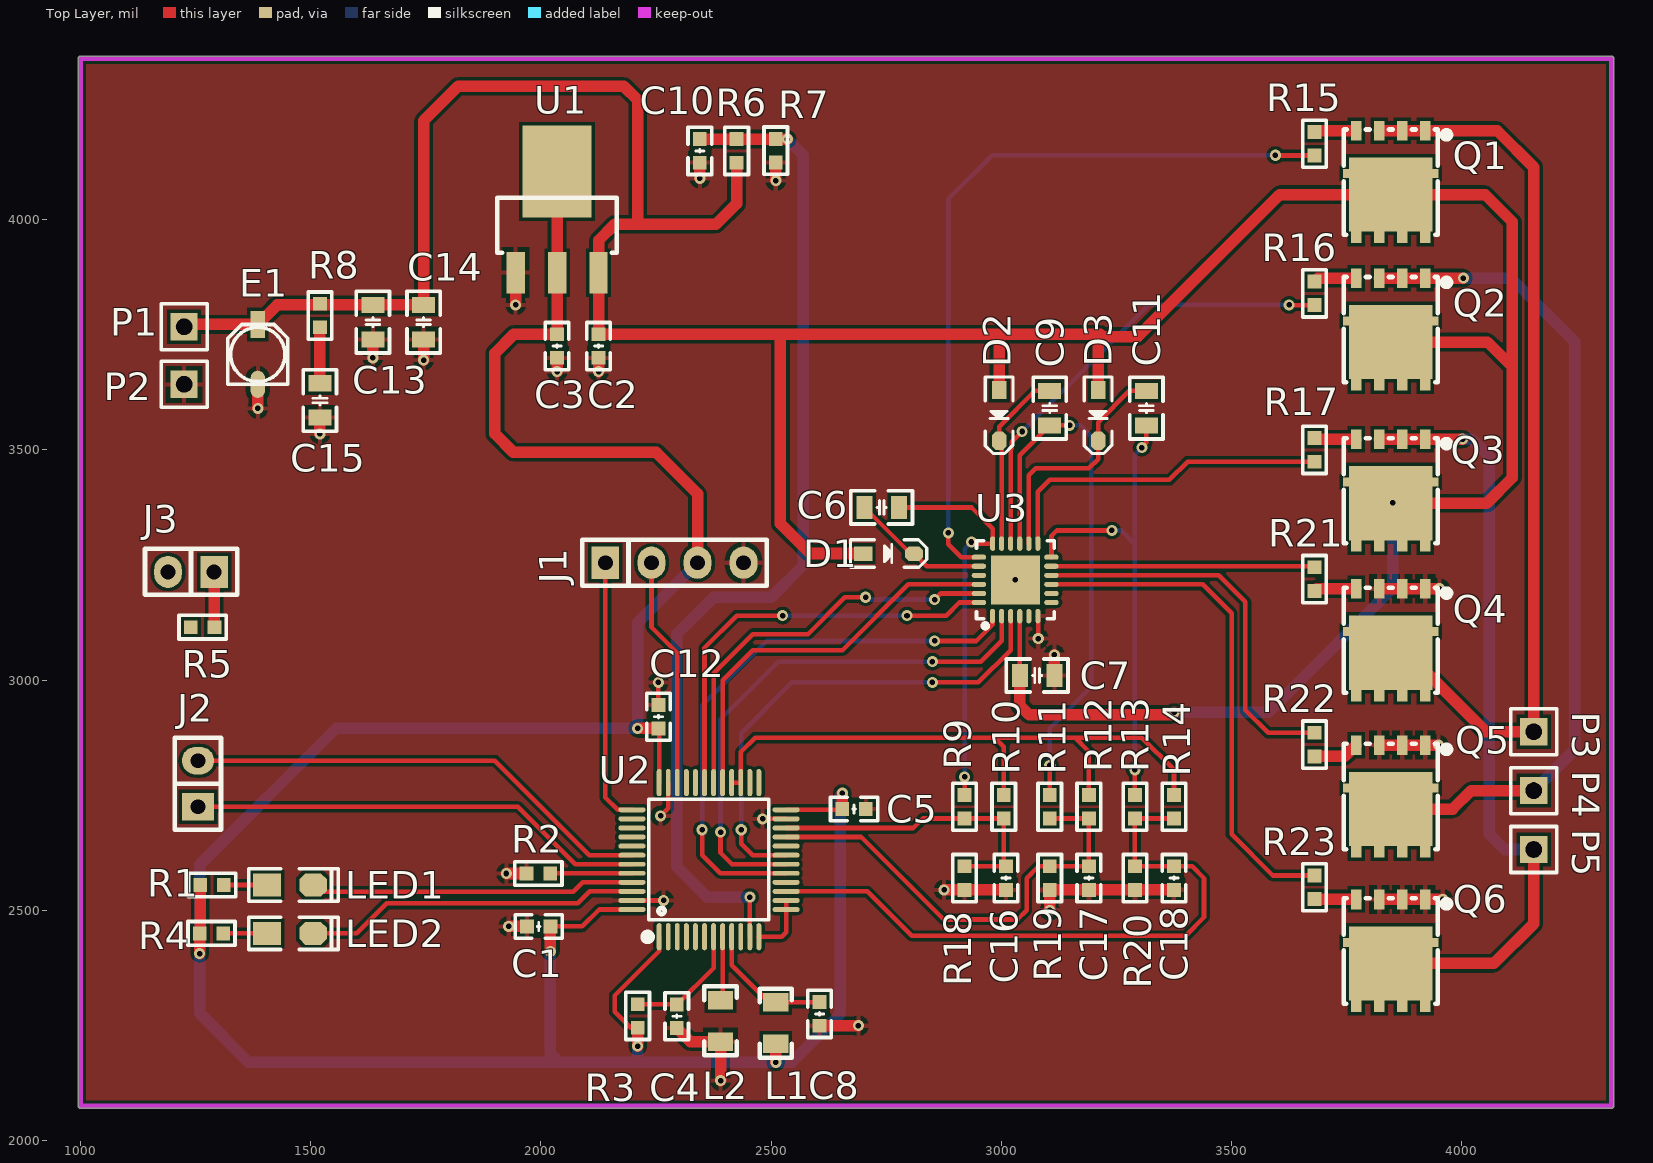
[diagram p0: Top Layer view]
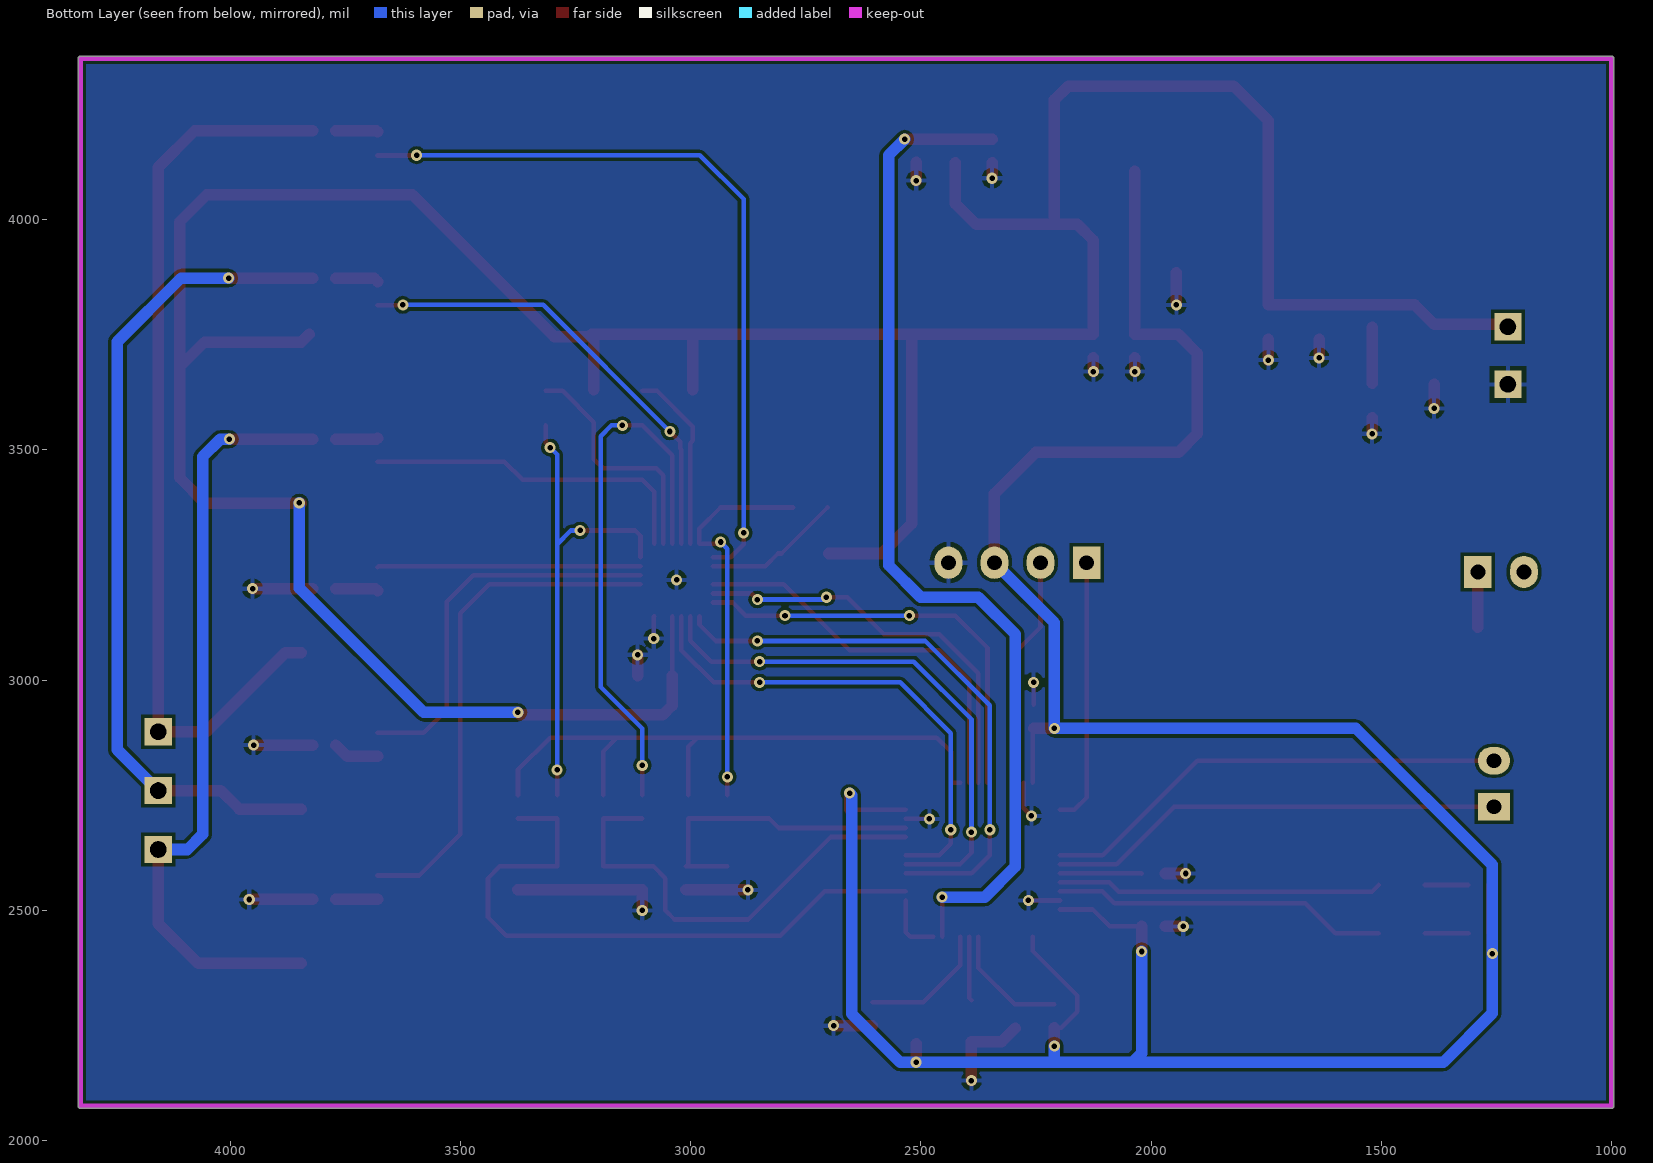
[diagram p1: Bottom Layer view, seen from below]
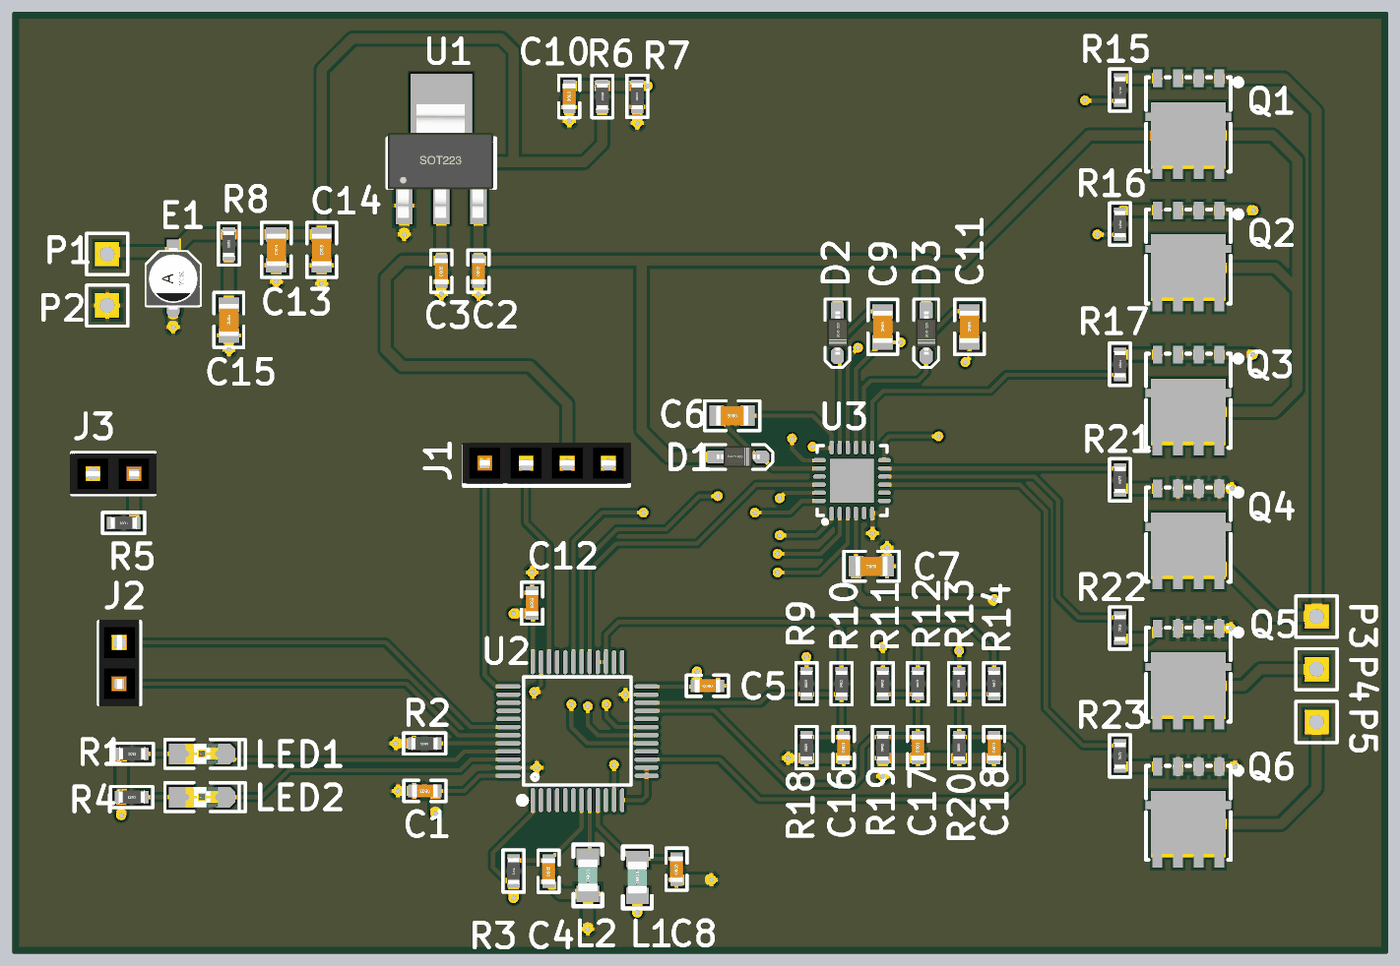
[diagram p2: 3D render of the assembled board from above, using the file's embedded part models]
# Altium PCB MISC82526.PcbDoc
Units mil, origin at the board's own origin, x right, y up, seen from the top; angles counter-clockwise.
Board outline 3335.03 x 2285.03 mil, 2 copper layers (Top Layer, Bottom Layer); 66 components, 53 nets, 254 pads, 58 vias.

## Layer stack, top to bottom (the 12.6 mil dielectric is the usual default, probably not edited)
Top Solder: solder mask 0.4, Solder Resist, Dk 3.5
Top Layer: signal copper 1.4
Dielectric 1: dielectric 12.6, FR-4, Dk 4.8
Bottom Layer: signal copper 1.4
Bottom Solder: solder mask 0.4, Solder Resist, Dk 3.5

## Board outline
1000,2069.99 cw(c1000,2075) 994.99,2075 994.99,4350 cw(c1000,4350) 1000,4355.02 4325,4355.02 cw(c4325,4350) 4330.02,4350 4330.02,2075 cw(c4325,2075) 4325,2069.99

## Design rules (kind name [scope] priority, off if disabled: settings)
Clearance [All] p1: gap=7
MinimumSolderMaskSliver [All] p1: minsoldermaskwidth=0
PolygonConnect [All] p1: connectstyle=Relief reliefconductorwidth=10 reliefentries=4 polygonreliefangle="90 Angle" airgapwidth=10
RoutingVias [All] p1: holewidth=28 width=50 viastyle="Through Hole" minholewidth=28 minwidth=50 maxholewidth=28 maxwidth=50
SilkToSilkClearance [All] p1: silktosilkclearance=0
SilkToSolderMaskClearance [IsPad] p1: minsilkscreentomaskgap=0 clearancetoexposedcopper=TRUE
SolderMaskExpansion [All] p1: expansion=4
Width [All] p1: maxlimit=30 minlimit=10 preferedwidth=10
27 further rules are at their usual default settings.

## Components (designator, comment, footprint, x,y, rotation, side; value= is the part's Value field where it differs from the comment)
C1 "100nF" "C 0603_L" 1995,2465 r180 top
C2 "10uF" "C 0603_L" 2125,3725.59 r90 top
C3 "100nF" "C 0603_L" 2035,3725.59 r90 top
C4 "100nF" "C 0603_L" 2295,2270 r90 top
C5 "100nF" "C 0603_L" 2680,2720 r180 top
C6 "4.7uF" "C 0805_L" 2740,3375 r180 top
C7 "22uF" "C 0805_L" 3077.6,3010 r180 top
C8 "100nF" "C 0603_L" 2605,2275 r90 top
C9 "4.7uF" "C 0805_L" 3105,3590.69 r90 top
C10 "100nF" "C 0603_L" 2345,4149.41 r90 top
C11 "4.7uF" "C 0805_L" 3315,3590.69 r90 top
C12 "100nF" "C 0603_L" 2255,2920.59 r90 top
C13 "22uF" "C 0805_L" 1635,3777.4 r90 top
C14 "22uF" "C 0805_L" 1745,3777.4 r90 top
C15 "10uF" "C 0805_L" 1520,3607.4 r90 top
C16 "100nF" "C 0603_L" 3010,2570 r90 top
C17 "100nF" "C 0603_L" 3190,2570 r90 top
C18 "100nF" "C 0603_L" 3375,2570 r90 top
D1 "B5819WS" SOD-323 2755,3275 r0 top
D2 "B5819WS" SOD-323 2995,3575.12 r270 top
D3 "B5819WS" SOD-323 3210,3575.12 r270 top
E1 "470uF" "CM A(3*5.4)" 1385,3707.4 r90 top
J1 "Female HDR1X4" Fe-HDR1X4/2.54-S 2140,3255 r90 top
J2 "Female HDR1X2" Fe-HDR1X2/2.54-S 1255,2725 r90 top
J3 "XH-2AW" Fe-HDR1X2/2.54-S 1290,3235 r180 top
L1 "10uH" "L 0805" 2510,2255 r90 top
L2 "10uH" "L 0805" 2390,2260 r90 top
LED1 "Red" "LED 0805G" 1455,2555 r0 top
LED2 "Red" "LED 0805G" 1455,2450 r0 top
P1 "HDR1X1" HDR1X1 1225,3767.4 r0 top
P2 "HDR1X1" HDR1X1 1225,3642.4 r0 top
P3 "HDR1X1" HDR1X1 4156.15,2887.87 r270 top
P4 "HDR1X1" HDR1X1 4156.15,2760 r270 top
P5 "HDR1X1" HDR1X1 4156.15,2632.12 r270 top
Q1 "WSD3095DN56" PDFN-8_L5.2-W5.9-P1.27-LS6.2-BL 3855,4085 r180 top
Q2 "WSD3095DN56" PDFN-8_L5.2-W5.9-P1.27-LS6.2-BL 3855,3764.65 r180 top
Q3 "WSD3095DN56" PDFN-8_L5.2-W5.9-P1.27-LS6.2-BL 3855,3414.75 r180 top
Q4 "WSD3095DN56" PDFN-8_L5.2-W5.9-P1.27-LS6.2-BL 3855,3090 r180 top
Q5 "WSD3095DN56" PDFN-8_L5.2-W5.9-P1.27-LS6.2-BL 3855,2750.41 r180 top
Q6 "WSD3095DN56" PDFN-8_L5.2-W5.9-P1.27-LS6.2-BL 3855,2415 r180 top
R1 "1K" "R 0603_L" 1285.59,2555 r180 top
R2 "10K" "R 0603_L" 1994.41,2580 r180 top
R3 "10K" "R 0603_L" 2210,2270.59 r270 top
R4 "2.7K" "R 0603_L" 1284.41,2450 r180 top
R5 "100" "R 0603_L" 1265,3115 r180 top
R6 "47K" "R 0603_L" 2425,4149.41 r270 top
R7 "10K" "R 0603_L" 2510,4150 r90 top
R8 "2" "R 0603_L" 1519.99,3791.82 r90 top
R9 "10K" "R 0603_L" 2920,2725 r90 top
R10 "1K" "R 0603_L" 3005,2725 r90 top
R11 "10K" "R 0603_L" 3105,2725 r90 top
R12 "1K" "R 0603_L" 3190,2725 r90 top
R13 "10K" "R 0603_L" 3290,2725 r90 top
R14 "1K" "R 0603_L" 3375,2725 r90 top
R15 "4.7" "R 0603_L" 3680.01,4165 r270 top
R16 "4.7" "R 0603_L" 3680.01,3840 r270 top
R17 "4.7" "R 0603_L" 3680.01,3500 r270 top
R18 "1K" "R 0603_L" 2920,2570 r90 top
R19 "1K" "R 0603_L" 3105,2570 r90 top
R20 "1K" "R 0603_L" 3290,2570 r90 top
R21 "4.7" "R 0603_L" 3680,3219.41 r90 top
R22 "4.7" "R 0603_L" 3680,2860 r90 top
R23 "4.7" "R 0603_L" 3680,2550 r90 top
U1 "AMS1117" SOT223 2035,3885 r0 top
U2 "CH32V203C8T6" LQFP-48_L7.0-W7.0-P0.50-LS9.0-BL 2365,2610 r0 top
U3 "FD6288Q_C7466367" QFN-24_L4.0-W4.0-P0.50-BL-EP2.7 3030,3210 r0 top

## Footprints (in the part's own frame and the unit in brackets; to place one, negate y for a bottom-side part, rotate by r counter-clockwise, add the part's x,y. Pads: shape width x height; smd on the part's side, far side on the other; paste and mask are expansions set on the pad)
"C 0603_L" [mil] "无极性贴片电容"
  rect 30x30 smd: 1(-25.59,0) 2(25.59,0)
  silkscreen extent -51,-26 51,26, body extent -31,-16 31,16, height 32
"C 0805_L" [mil] "无极性贴片电容"
  rect 35x50 smd: 1(-37.4,0) 2(37.4,0)
  silkscreen extent -67,-36 67,36, body extent -39,-24 39,24, height 20
"CM A(3*5.4)" [mm] "贴片电解电容，直径3mm，高5.4mm"
  rect 1.5x0.8 smd: 1(1.651,0)
  oval 1.5x0.8 smd: 2(-1.65,0)
  silkscreen extent -1.65,-1.65 1.65,1.65, body extent -1.9,-1.65 1.9,1.65, height 5.4
Fe-HDR1X2/2.54-S [mil] "Connector; Header; 2x2 Position"
  rect 60x70 hole 32: 1(0,0)
  oval 60x70 hole 32: 2(100,0)
  silkscreen extent -50,-50 150,50, body extent -55,-48 155,50, height 335
Fe-HDR1X4/2.54-S [mil]
  rect 70x60 hole 32: 1(0,0)
  oval 70x60 hole 32: 2(0,-100) 3(0,-200) 4(0,-300)
  silkscreen extent -50,-350 50,50, body extent -44,-355 54,55, height 335
HDR1X1 [mm]
  rect 1.5x1.5 hole 0.9 slot 0.905 at 0 deg paste+0 mask+0.051: 1(0,0)
  silkscreen extent -1.27,-1.27 1.27,1.27
"L 0805" [mil] "小功率贴片电感"
  rect 40x55 smd: 1(-45,0) 2(45,0)
  silkscreen extent -75,-35 75,35, body extent -39,-24 39,24, height 35
"LED 0805G" [mil] "绿色0805LED"
  rect 60x50 smd: 1(-50,0)
  oct 60x50 smd: 2(50,0)
  silkscreen extent -90,-35 105,35, body extent -39,-25 39,25, height 32
LQFP-48_L7.0-W7.0-P0.50-LS9.0-BL [mm]
  oval 0.27x1.5 smd paste+0 mask+0.051: 1(-2.75,-4.25) 2(-2.25,-4.25) 3(-1.75,-4.25) 4(-1.25,-4.25) 5(-0.75,-4.25) 6(-0.25,-4.25) 7(0.25,-4.25) 8(0.75,-4.25) 9(1.25,-4.25) 10(1.75,-4.25) 11(2.25,-4.25) 12(2.75,-4.25) 25(2.75,4.25) 26(2.25,4.25) 27(1.75,4.25) 28(1.25,4.25) 29(0.75,4.25) 30(0.25,4.25) 31(-0.25,4.25) 32(-0.75,4.25) 33(-1.25,4.25) 34(-1.75,4.25) 35(-2.25,4.25) 36(-2.75,4.25)
  oval 1.5x0.27 smd paste+0 mask+0.051: 13(4.25,-2.75) 14(4.25,-2.25) 15(4.25,-1.75) 16(4.25,-1.25) 17(4.25,-0.75) 18(4.25,-0.25) 19(4.25,0.25) 20(4.25,0.75) 21(4.25,1.25) 22(4.25,1.75) 23(4.25,2.25) 24(4.25,2.75) 37(-4.25,2.75) 38(-4.25,2.25) 39(-4.25,1.75) 40(-4.25,1.25) 41(-4.25,0.75) 42(-4.25,0.25) 43(-4.25,-0.25) 44(-4.25,-0.75) 45(-4.25,-1.25) 46(-4.25,-1.75) 47(-4.25,-2.25) 48(-4.25,-2.75)
  silkscreen extent -3.59,-4.46 3.3,3.34
PDFN-8_L5.2-W5.9-P1.27-LS6.2-BL [mm]
  rect 0.58x1.079 smd paste-100 mask+0.05: 1(-1.668,-2.757) 2(-0.398,-2.757) 3(0.872,-2.757) 4(2.142,-2.757)
  rect 0.58x1.08 smd paste-100 mask+0.05: 5(2.147,2.912) 6(0.878,2.912) 7(-0.392,2.912) 8(-1.662,2.912)
  rect 0.95x0.5 smd paste-100 mask+0.05: 9(-1.932,-0.387) 9(2.407,-0.387)
  rect 4.6x4.1 smd paste-100 mask+0.05: 9(0.237,0.773)
  silkscreen extent -2.96,-2.82 2.84,2.98
QFN-24_L4.0-W4.0-P0.50-BL-EP2.7 [mm]
  oval 0.28x0.8 smd paste+0 mask+0.051: 1(-1.25,-1.803) 2(-0.75,-1.803) 3(-0.25,-1.803) 4(0.25,-1.803) 5(0.75,-1.803) 6(1.25,-1.803) 13(1.25,2.197) 14(0.75,2.197) 15(0.25,2.197) 16(-0.25,2.197) 17(-0.75,2.197) 18(-1.242,2.197)
  oval 0.8x0.28 smd paste+0 mask+0.051: 7(2,-1.053) 8(2,-0.553) 9(2,-0.053) 10(2,0.447) 11(2,0.947) 12(2,1.447) 19(-2,1.447) 20(-2,0.947) 21(-2,0.447) 22(-2,-0.053) 23(-2,-0.553) 24(-2,-1.053)
  rect 2.7x2.7 smd paste+0 mask+0.051: 25(0.012,0.197)
  silkscreen extent -2.14,-2.6 2.16,2.35
"R 0603_L" [mil] "1/10W贴片电阻"
  rect 30x30 smd: 1(-25.59,0) 2(25.59,0)
  silkscreen extent -51,-26 51,26, body extent -31,-16 32,16, height 16
SOD-323 [mm] "1.8x1.3X0.9mm（长宽高，不包括引脚）"
  rect 1x0.8 smd: 1(-1.4,0)
  oct 1x0.8 smd: 2(1.4,0)
  silkscreen extent -2.11,-0.76 2.11,0.76, body extent -1.34,-0.63 1.31,0.67, height 1
SOT223 [mil]
  rect 40x90 smd: 1(-90,0) 2(0,0) 3(90,0)
  rect 150x200 smd: 2(0,220)
  silkscreen extent -130,43 130,163, body extent -130,-30 126,246, height 65

## Part data
C1 C2 C3 C4 C5 C6 C7 C8 C9 C10 C11 C12 C13 C14 C15 C16 C17 C18: library part C, "SMD capacitor"
D1 D2 D3: library part 1N5819, "Schottky diode"
E1: library part CE_SMD, "SMD electrolytic capacitor"
J3: library part "Female HDR1X2"
L1 L2: library part L, "Low-power SMD inductor"
LED1 LED2: library part LED-SMD, "SMD LED"
R1 R2 R3 R4 R5 R6 R7 R8 R9 R10 R11 R12 R13 R14 R15 R16 R17 R18 R19 R20 R21 R22 R23: library part R, "SMD resistor"
U1: "Three-terminal voltage regulator"

## Via types
v1: diameter 24, hole 12, Top Layer to Bottom Layer, 58 vias

## Nets (pads, with @x,y where several pads share a name; then routed paths per layer and width w, separated by ;. In a path a pad name is that pad's centre, name@x,y a point inside that pad or via, vN(x,y) a via of type N, cw(c..) or ccw(c..) an arc to the next point about the centre after c; other vN are vias at no path point)
3.3V: C1.1 C3.2 C5.2 C12.1 J1.3 L1.1 R1.2 R3.2 R4.2 U1.2 U2.1 U2.24 U2.36 U2.48 | length 6444.5
  Top Layer w10: C1.1 2090,2465 2126.73,2501.73 U2.48 ; R3.2 2195,2245 2160,2280 2160,2315 2256.73,2411.73 U2.1 ; C12.1 2256.73,2893.27 U2.36 ; U2.24 2652.68,2718.27 C5.2
  Top Layer w25: v1(1258.82,2406.18) R4.2 1260,2451.18 R1.2 ; v1(2020.59,2410.59) C1.1 ; U1.2@2035,4105 2035,3885 C3.2 1941.18,3751.18 1900,3710 1900,3535 1940,3495 2250,3495 2340,3405 J1.3 ; v1(2210,2205) R3.2 ; v1(2210,2895) C12.1 ; v1(2510,2170) L1.1 ; C5.2 v1(2654.41,2754.41)
  Bottom Layer w25: v1(2020.59,2410.59) 2020.59,2189.41 2040,2170 ; v1(2210,2205) 2210,2175 2205,2170 ; J1.3 2210,3125 v1(2210,2895) 1555,2895 1258.82,2598.82 v1(1258.82,2406.18) 1258.82,2276.18 1365,2170 2040,2170 ; v1(2654.41,2754.41) 2650,2750 2650,2275 2545,2170 v1(2510,2170) 2205,2170 ; 2040,2170 2205,2170
ABMF: C16.2 R9.1 R10.1 R18.2 U2.22 | length 677.1
  Top Layer w10: U2.22 2808.9,2678.9 2829.41,2699.41 R9.1 R10.1 3005,2600.58 C16.2 R18.2
BAT_ADC: C10.2 R6.1 R7.2 U2.11 | length 2243.6
  Top Layer w10: U2.11 v1(2453.58,2528.58)
  Top Layer w25: C10.2 R6.1 v1(2535,4175)
  Bottom Layer w25: v1(2453.58,2528.58) 2361.42,2528.58 2295,2595 2295,3100 2375,3180 2500,3180 2570,3250 2570,4140 v1(2535,4175)
BBMF: C17.2 R11.1 R12.1 R19.2 U2.21 | length 1009.6
  Top Layer w10: U2.21 2695.79,2659.21 2875,2480 3035,2480 3055,2500 3055,2570 3080.59,2595.59 R19.2 C17.2 R12.1 R11.1
CBMF: C18.2 R13.1 R14.1 R20.2 U2.15 | length 1398.5
  Top Layer w10: U2.15 2708.9,2541.1 2805,2445 3400,2445 3440,2485 3440,2570 3414.41,2595.59 C18.2 R20.2 R13.1 R14.1
CLK: J1.1 U2.37 | length 578.8
  Top Layer w10: J1.1 2140,2745 2166.73,2718.27 U2.37
CMPO: U2.12 U2.13 U2.14 | length 132.1
  Top Layer w10: U2.12 2522.68,2442.68 2532.32,2452.32 U2.13 U2.14
DIO: J1.2 U2.34 | length 500.9
  Top Layer w10: J1.2 2240,3115 2296.1,3058.9 U2.34
ERR: LED1.2 U2.45 | length 707.5
  Top Layer w10: LED1.2 1520,2540 2070,2540 2090.79,2560.79 U2.45
GND: C1.2 C2.1 C3.1 C4.1 C5.1 C7.1 C8.1 C10.1 C12.2 C13.1 C14.1 C15.1 C16.1 C17.1 C18.1 E1.2 J1.4 L2.1 P2.1 Q4.1 Q4.2 Q4.3 Q5.1 Q5.2 Q5.3 Q6.1 Q6.2 Q6.3 R2.2 R7.1 R18.1 R19.1 R20.1 U1.1 U2.23 U2.35 U2.47 U3.6 U3.25 | length 1923.2
  Top Layer w10: U2.47 v1(2266.42,2521.42) ; C12.2 v1(2255,2995) ; v1(2260,2705) 2276.42,2721.42 U2.35 ; v1(2481.42,2698.58) U2.23 ; U3.6 3080,3138.24 v1(3080,3090)
  Top Layer w25: v1(1385,3590) E1.2 ; v1(1520,3535) C15.1 ; v1(1635,3700) C13.1 ; v1(1745,3695) C14.1 ; v1(1925,2580) R2.2 ; v1(1930,2465) C1.2 ; v1(1945,3815) U1.1 ; v1(2035,3670) C3.1 ; v1(2125,3670) C2.1 ; C4.1 2324.41,2215 L2.1 v1(2390,2130) ; v1(2345,4090) C10.1 ; v1(2510,4085) R7.1 ; C8.1 v1(2689.41,2249.41) ; v1(2875.59,2544.41) R18.1 C16.1 ; v1(3105,2500) R19.1 C17.1 R20.1 C18.1 ; C7.1 v1(3115,3055) ; Q6.3 Q6.2 Q6.1 v1(3958.55,2523.55) ; Q5.3 Q5.2 Q5.1 v1(3948.96,2858.96) ; Q4.3 Q4.2 Q4.1 v1(3951.45,3198.55)
  other v1: 3030.49,3217.76
HOA: R15.2 U3.19 | length 1662.5
  Top Layer w10: v1(2885,3320) 2885,3295 2913.02,3266.98 U3.19 ; v1(3595,4140) 3595.59,4139.41 R15.2
  Bottom Layer w10: v1(2885,3320) 2885,4045 2980,4140 v1(3595,4140)
HOB: R16.2 U3.16 | length 1002.9
  Top Layer w10: U3.16 3020.17,3500.64 3022.75,3503.22 3022.75,3517.75 v1(3045,3540) ; v1(3625,3815) 3625.59,3814.41 R16.2
  Bottom Layer w10: v1(3045,3540) 3320,3815 v1(3625,3815)
HOC: R17.2 U3.13 | length 740.5
  Top Layer w10: U3.13 3079.22,3409.22 3105,3435 3365,3435 3404.41,3474.41 R17.2
LOA: R21.2 U3.11 | length 572.2
  Top Layer w10: U3.11 3677.71,3247.3 R21.2
LOB: R22.2 U3.10 | length 850.6
  Top Layer w10: U3.10 3472.39,3227.61 3530,3170 3530,2935 3579.41,2885.59 R22.2
LOC: R23.2 U3.9 | length 1114.4
  Top Layer w10: U3.9 3437.07,3207.93 3500,3145 3500,2665 3589.41,2575.59 R23.2
MID: R10.2 R12.2 R14.2 U2.27 U2.28 | length 1393.2
  Top Layer w10: U2.28 U2.27 2433.9,2843.9 2465,2875 2985,2875 ; R10.2 3005,2855 2985,2875 ; R12.2 3190,2845 3160,2875 ; R14.2 3375,2805 3305,2875 3160,2875 ; 2985,2875 3160,2875
NetC6_2: C6.2 D1.2 U3.20 | length 301.6
  Top Layer w10: C6.2 2802.6,3275 D1.2 2837.82,3247.3 U3.20
NetC8_2: C8.2 L1.2 U2.9 | length 286.4
  Top Layer w10: U2.9 2414.21,2380.79 2495,2300 L1.2 2604.42,2300 C8.2
NetC9_2: C9.2 D2.2 U3.17 | length 398.1
  Top Layer w10: U3.17 3000.48,3514.52 D2.2 2995,3550 3073.09,3628.09 C9.2
NetC11_2: C11.2 D3.2 U3.14 | length 526.4
  Top Layer w10: U3.14 3059.54,3444.54 3075,3460 3190,3460 3210,3480 D3.2 3210,3560 3278.09,3628.09 C11.2
NetC15_2: C15.2 R8.1 | length 121.4
  Top Layer w25: C15.2 R8.1
NetJ3_1: J3.1 R5.1 | length 120.2
  Top Layer w25: J3.1 1290.59,3234.41 R5.1
NetJ3_2: J3.2
NetL2_2: L2.2 U2.8 | length 139.6
  Top Layer w10: L2.2 2394.53,2309.53 U2.8
NetLED1_1: LED1.1 R1.1 | length 93.8
  Top Layer w10: R1.1 LED1.1
NetLED2_1: LED2.1 R4.1 | length 95
  Top Layer w10: R4.1 LED2.1
NetP3_1: P3.1 Q1.1 Q1.2 Q1.3 Q4.5 Q4.6 Q4.7 Q4.8 Q4.9 | length 1976.1
  Top Layer w25: Q1.3 Q1.2 Q1.1 4076.45,4193.55 4156.15,4113.85 P3.1 4052.13,2887.87 3880.41,3059.59 Q4.9@3845.65,3059.59
NetP4_1: P4.1 Q2.1 Q2.2 Q2.3 Q5.5 Q5.6 Q5.7 Q5.8 Q5.9 | length 1820.5
  Top Layer w25: Q2.3 Q2.2 Q2.1 v1(4003.2,3873.2) ; Q5.9@3845.65,2720 3980,2720 4020,2760 P4.1
  Bottom Layer w25: v1(4003.2,3873.2) 4106.8,3873.2 4245,3735 4245,2848.85 P4.1
NetP5_1: P5.1 Q3.1 Q3.2 Q3.3 Q6.5 Q6.6 Q6.7 Q6.8 Q6.9 | length 1692.3
  Top Layer w25: Q3.3 Q3.2 Q3.1 v1(4001.7,3523.3) ; Q6.9@3845.65,2384.59 4069.59,2384.59 4156.15,2471.15 P5.1
  Bottom Layer w25: v1(4001.7,3523.3) 4021.7,3523.3 4060,3485 4060,2665 4092.88,2632.12 P5.1
NetQ1_4: Q1.4 R15.1 | length 91.9
  Top Layer w25: R15.1 3682.95,4193.55 Q1.4
NetQ2_4: Q2.4 R16.1 | length 93.8
  Top Layer w25: R16.1 3687.61,3873.2 Q2.4
NetQ3_4: Q3.4 R17.1 | length 91.6
  Top Layer w25: R17.1 3682.3,3523.3 Q3.4
NetQ4_4: Q4.4 R21.1 | length 92.6
  Top Layer w25: R21.1 3684.73,3198.55 Q4.4
NetQ5_4: Q5.4 R22.1 | length 100.8
  Top Layer w25: R22.1 3746.1,2834.41 Q5.4
NetQ6_4: Q6.4 R23.1 | length 91
  Top Layer w25: R23.1 3769.79,2524.41 Q6.4
NetR2_1: R2.1 U2.44 | length 177.9
  Top Layer w10: R2.1 2020.47,2580.47 U2.44
NetR5_2: R5.2
NRST: C4.2 R3.1 U2.7 | length 265.8
  Top Layer w10: R3.1 2294.41,2296.18 C4.2 2295.59,2295.59 2374.84,2374.84 U2.7
PWMAH: U2.29 U3.22 | length 865.3
  Top Layer w10: U2.29 2394.53,2999.53 2460,3065 2655,3065 2797.93,3207.93 U3.22
PWMAL: U2.17 U3.1 | length 1245.5
  Top Layer w10: v1(2350,2675) 2350,2620 2389.53,2580.47 U2.17 ; v1(2855,3085) 2945,3085 2980.8,3120.8 U3.1
  Bottom Layer w10: v1(2350,2675) 2350,2945 2490,3085 v1(2855,3085)
PWMBH: U2.30 U3.23 | length 889.9
  Top Layer w10: U2.30 2374.84,3014.84 2460,3100 2580,3100 2660,3180 v1(2705,3180) ; v1(2855,3175) 2868.24,3188.24 U3.23
  Bottom Layer w10: v1(2705,3180) 2710,3175 v1(2855,3175)
PWMBL: U2.18 U3.2 | length 1177.2
  Top Layer w10: v1(2390,2670) 2390,2625 2414.84,2600.16 U2.18 ; v1(2850,3040) 2955,3040 3000.48,3085.48 U3.2
  Bottom Layer w10: v1(2390,2670) 2390,2915 2515,3040 v1(2850,3040)
PWMCH: U2.31 U3.24 | length 929.7
  Top Layer w10: U2.31 2355.16,3070.16 2425,3140 v1(2525,3140) ; v1(2795,3140) 2880,3140 2908.56,3168.56 U3.24
  Bottom Layer w10: v1(2525,3140) v1(2795,3140)
PWMCL: U2.19 U3.3 | length 1081.4
  Top Layer w10: v1(2435,2675) 2435,2645 2460.16,2619.84 U2.19 ; v1(2850,2995) 2950,2995 3020.17,3065.17 U3.3
  Bottom Layer w10: v1(2435,2675) 2435,2885 2545,2995 v1(2850,2995)
PWMIN: U2.38
RUN: LED2.2 U2.46 | length 730.4
  Top Layer w10: LED2.2 1600,2450 1665,2515 2080,2515 2106.1,2541.1 U2.46
RX: J2.1 U2.43 | length 994.4
  Top Layer w10: J2.1 1950,2725 2074.84,2600.16 U2.43
TX: J2.2 U2.42 | length 1027.7
  Top Layer w10: J2.2 1900,2825 2105.16,2619.84 U2.42
VBAT: C2.2 C7.2 C13.2 C14.2 D1.1 D2.1 D3.1 E1.1 P1.1 Q1.5 Q1.6 Q1.7 Q1.8 Q1.9 Q2.5 Q2.6 Q2.7 Q2.8 Q2.9 Q3.5 Q3.6 Q3.7 Q3.8 Q3.9 R6.2 R8.2 U1.3 U3.4 | length 7815
  Top Layer w10: U3.4 3039.85,3010.35 C7.2
  Top Layer w25: P1.1 1230,3772.4 E1.1 1427.4,3814.8 C13.2 C14.2 1745,4215 1820,4290 2180,4290 2210,4260 2210,3990 ; R6.2 2425,4035 2380,3990 2210,3990 ; D1.1 2585,3275 2520,3340 2520,3751.18 ; D2.1 2995,3746.18 3000,3751.18 ; C7.2 3040.2,2944.8 3060,2925 3370,2925 v1(3375,2930) ; D3.1 3210,3746.18 ; Q2.9@3828.71,3751.18 3845.65,3734.24 4055.76,3734.24 4110,3680 ; Q3.9@3845.65,3384.34 4054.34,3384.34 4110,3440 4110,3680 ; 2210,3990 2160,3990 2125,3955 U1.3 C2.2 2520,3751.18 ; 2520,3751.18 3000,3751.18 ; 3000,3751.18 3215,3751.18 3210,3746.18 ; 3210,3746.18 3296.18,3746.18 3604.59,4054.59 3845.65,4054.59 4050.41,4054.59 4110,3995 4110,3680
  Bottom Layer w25: v1(3375,2930) 3580,2930 3850,3200 v1(3850,3385)
VSA: C6.1 R9.2 U3.18 | length 858.4
  Top Layer w10: C6.1 2935,3375 2981.11,3328.89 U3.18 2938.5,3296.5 v1(2935,3300) ; R9.2 v1(2920,2790)
  Bottom Layer w10: v1(2920,2790) 2920,3285 v1(2935,3300)
VSB: C9.1 R11.2 U3.15 | length 1200.1
  Top Layer w10: U3.15 3039.85,3488.13 C9.1 v1(3148.28,3553.28) ; R11.2 v1(3105,2815)
  Bottom Layer w10: v1(3105,2815) 3105,2895 3195,2985 3195,3530 3171.72,3553.28 v1(3148.28,3553.28)
VSC: C11.1 R13.2 U3.12 | length 1058.2
  Top Layer w10: U3.12 3108.74,3313.74 3120,3325 v1(3240,3325) ; R13.2 v1(3290,2805) ; v1(3305,3505) 3315,3515 C11.1
  Bottom Layer w10: v1(3240,3325) 3260,3325 3290,3295 ; v1(3290,2805) 3290,3295 ; v1(3305,3505) 3290,3490 3290,3295
pads on no net: U2.2 U2.3 U2.4 U2.5 U2.6 U2.10 U2.16 U2.20 U2.25 U2.26 U2.32 U2.33 U2.39 U2.40 U2.41 U3.5 U3.7 U3.8 U3.21

## Polygon pours and split planes (outlines as drawn)
GND on Bottom Layer "D" (solid, remove dead copper, pour order 2): 730,4480 4660,4480 4710,4530 4440,4260 4440,1665 970,1665 910,1725
GND on Top Layer "D" (solid, remove dead copper, pour order 4): 795,4475 830,4440 4585,4440 4585,2280 4470,2165 4425,2120 4425,1815 1045,1815 855,2005

## Keep-outs
Keep-Out Layer:
  lines w10: 1000,3890 1000,4350 4125,4350 4325,4350 4325,2075 1175,2075 1000,2075 1000,3950